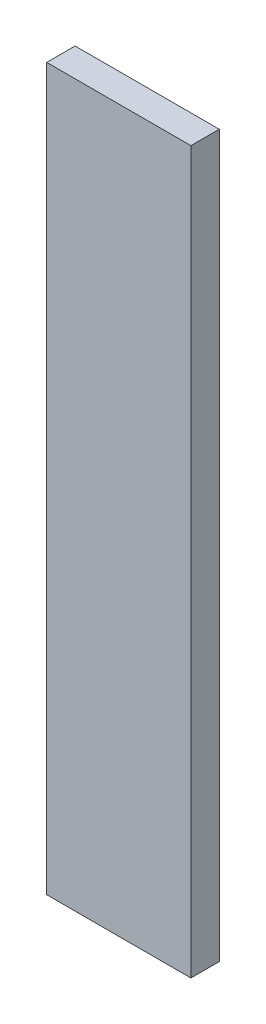
SolidWorks part; units mm, degrees
material "普通碳钢"
ref_plane "Front Plane" through (0, 0, 0) normal (0, 0, 1) x (1, 0, 0)
ref_plane "Top Plane" through (0, 0, 0) normal (0, 1, 0) x (1, 0, 0)
ref_plane "Right Plane" through (0, 0, 0) normal (1, 0, 0) x (0, 0, -1)
sketch "Sketch1" plane through (0, 0, 0) normal (0, 0, 1) x (1, 0, 0)
  line L1 (-25.4, 127) -> (25.4, 127)
  line L2 (-25.4, 127) -> (-25.4, -127)
  line L3 (-25.4, -127) -> (25.4, -127)
  line L4 (25.4, 127) -> (25.4, -127)
  dimension "D1" = 50.8
  dimension "D2" = 25.4
  dimension "D3" = 254
  dimension "D4" = 127
extrude "Boss-Extrude1" add sketch "Sketch1" along normal mid plane 10
